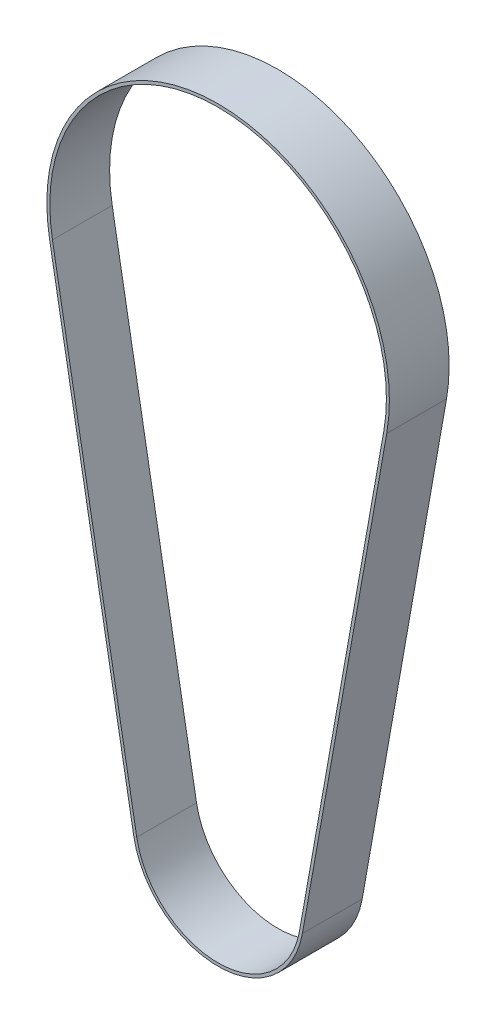
SolidWorks part; units mm, degrees
ref_plane "Front Plane" through (0, 0, 0) normal (0, 0, 1) x (1, 0, 0)
ref_plane "Top Plane" through (0, 0, 0) normal (0, 1, 0) x (1, 0, 0)
ref_plane "Right Plane" through (0, 0, 0) normal (1, 0, 0) x (0, 0, -1)
sketch "Sketch1" plane through (0, 0, 0) normal (0, 0, 1) x (1, 0, 0)
  line L0 (-28.2094, 76.995) -> (-14.1047, -2.5025)
  line L1 (28.2094, 76.995) -> (14.1047, -2.5025)
  line L2 (-27.7171, 77.0823) -> (-13.6124, -2.4152)
  line L3 (27.7171, 77.0823) -> (13.6124, -2.4152)
  arc A0 (-14.1047, -2.5025) -> (14.1047, -2.5025) centre (0, 0) ccw
  arc A1 (28.2094, 76.995) -> (-28.2094, 76.995) centre (0, 82) ccw
  arc A2 (-13.6124, -2.4152) -> (13.6124, -2.4152) centre (0, 0) ccw
  arc A3 (27.7171, 77.0823) -> (-27.7171, 77.0823) centre (0, 82) ccw
  dimension "D2" = 28.65
  dimension "D3" = 57.3
  dimension "D1" = 82
  dimension "D4" = 0.5
extrude "Boss-Extrude1" add sketch "Sketch1" along normal mid plane 10
